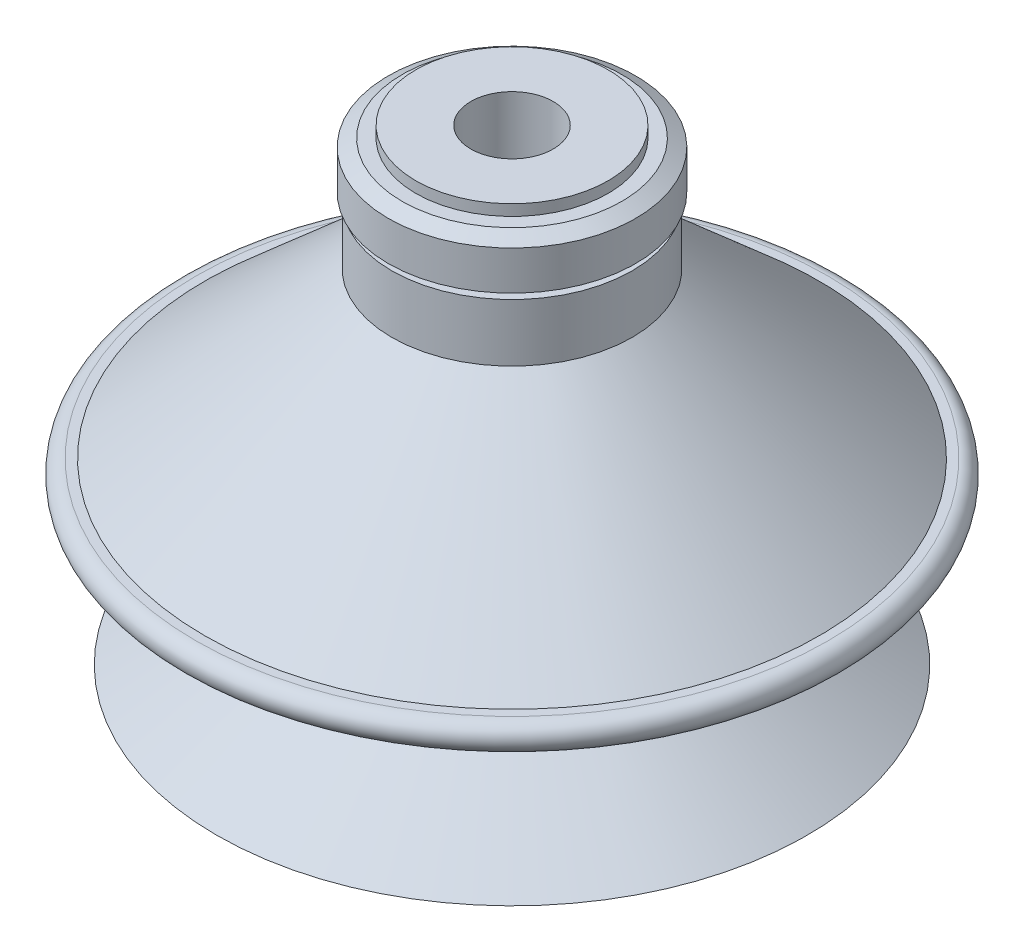
from build123d import *


with BuildPart() as part:
    # Sketch1 → Revolve1 (revolve)
    with BuildSketch(Plane.XY, mode=Mode.PRIVATE) as revolve1_sk:
        with BuildLine():
            Line((3, 0), (21.5, 0))
            Line((21.5, 0), (14.481102974, 4.822150816))
            ThreePointArc((14.481102974, 4.822150816), (14.13417871, 5.491793096), (14.498167484, 6.152315163))
            Line((14.498167484, 6.152315163), (21.957245997, 11))
            Line((21.957245997, 11), (23, 11))
            ThreePointArc((23, 11), (24, 12), (23, 13))
            Line((23, 13), (22.361328191, 13))
            Line((22.361328191, 13), (8.75, 25))
            Line((8.75, 25), (8.75, 29.2))
            Line((8.75, 29.2), (8, 29.2))
            Line((8, 29.2), (9, 29.777350269))
            Line((9, 29.777350269), (9, 32.622649731))
            Line((9, 32.622649731), (8, 33.2))
            Line((8, 33.2), (7, 33.2))
            Line((7, 33.2), (7, 34))
            Line((7, 34), (3, 34))
            Line((3, 34), (3, 0))
        make_face()
    revolve(revolve1_sk.sketch.rotate(Axis((0, 0, 0), (0, 1, 0)), 270), axis=Axis((0, 0, 0), (0, 1, 0)))


solid = part.part
